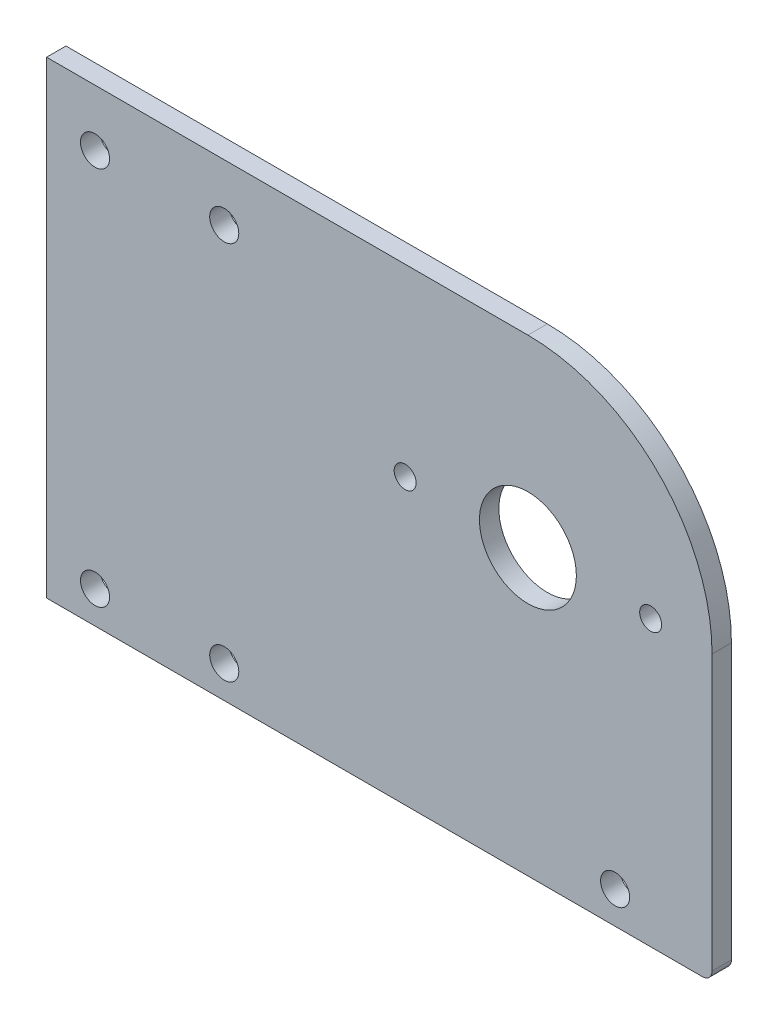
SolidWorks part; units mm, degrees
material "普通碳钢"
ref_plane "前视基准面" through (0, 0, 0) normal (0, 0, 1) x (1, 0, 0)
ref_plane "上视基准面" through (0, 0, 0) normal (0, 1, 0) x (1, 0, 0)
ref_plane "右视基准面" through (0, 0, 0) normal (1, 0, 0) x (0, 0, -1)
sketch "草图1" plane through (0, 0, 0) normal (0, 0, 1) x (1, 0, 0)
  line L0 (0, 72.5) -> (0, 0) construction
  line L1 (-103, 72.5) -> (103, 72.5)
  line L2 (-103, 72.5) -> (-103, -72.5)
  line L3 (-103, -72.5) -> (103, -72.5)
  line L4 (103, 72.5) -> (103, -72.5)
  line L5 (0, 0) -> (103, 0) construction
  dimension "D1" = 206
  dimension "D2" = 145
extrude "凸台-拉伸1" add sketch "草图1" along normal blind 6
sketch "草图2" plane through (0, 0, 6) normal (0, 0, 1) x (1, 0, 0)
  line L0 (103, 72.5) -> (-103, 72.5) construction
  line L1 (-103, -72.5) -> (-3, -72.5)
  line L2 (-103, -72.5) -> (-103, -7.5)
  line L3 (-103, -7.5) -> (-3, -7.5)
  line L4 (-3, -72.5) -> (-3, -7.5)
  dimension "D1" = 80
  dimension "D2" = 100
extrude "切除-拉伸1" [suppressed] cut sketch "草图2" against normal through all
sketch "草图3" plane through (0, 0, 6) normal (0, 0, 1) x (1, 0, 0)
  line L0 (103, 72.5) -> (-103, 72.5) construction
  line L1 (-103, 72.5) -> (-103, -72.5) construction
  circle A0 centre (-88, 55) radius 4.5
  circle A1 centre (-48, 55) radius 4.5
  circle A2 centre (-88, -62.5) radius 4.5
  circle A3 centre (-48, -62.5) radius 4.5
  dimension "D1" = 9
  dimension "D2" = 40
  dimension "D3" = 117.5
  dimension "D4" = 17.5
  dimension "D5" = 15
extrude "切除-拉伸2" cut sketch "草图3" against normal through all
sketch "草图4" plane through (0, 0, 6) normal (0, 0, 1) x (1, 0, 0)
  line L0 (103, 72.5) -> (-103, 72.5) construction
  line L2 (103, -72.5) -> (103, 72.5) construction
  circle A0 centre (46, 15.5) radius 15
  dimension "D1" = 30
  dimension "D3" = 57
  dimension "D2" = 57
extrude "切除-拉伸3" cut sketch "草图4" against normal through all
fillet "圆角1" radius 57 1 edges at (103, 72.5, 3)
fillet "圆角2" [suppressed] radius 10
fillet "圆角3" [suppressed] radius 10
sketch "草图5" plane through (0, 0, 6) normal (0, 0, 1) x (1, 0, 0)
  line L0 (46, 72.5) -> (-103, 72.5) construction
  line L1 (103, -72.5) -> (103, 15.5) construction
  circle A0 centre (88, 61) radius 2.75
  dimension "D1" = 11.5
  dimension "D2" = 5.5
  dimension "D3" = 15
extrude "切除-拉伸4" [suppressed] cut sketch "草图5" against normal through all
hole_wizard "M8 螺纹孔1" positions "草图7" profile "草图6" tap size "M8" standard "Gb" end condition through all
sketch "草图7" plane through (0, 0, 6) normal (0, 0, 1) x (1, 0, 0)
  line L0 (46, 41.9926) -> (46, 15.5) construction
  line L1 (46, 15.5) -> (88.8291, 15.5) construction
  point P0 (8, 15.5)
  dimension "D1" = 38
cosmetic thread "孔螺蚊线1" parameters "D2"=8
sketch "草图6" plane through (8, 15.5, 6) normal (1, 0, 0) x (0, -1, 0)
  line L0 (0, 0) -> (0, 6)
  line L1 (0, 6) -> (3.4, 6)
  line L2 (3.4, 6) -> (3.4, 0)
  line L5 (3.4, 0) -> (0, 0)
  line L11 (0, -6.35) -> (0, 107.95) construction
  dimension "通孔螺纹孔钻头直径" = 6.8
  dimension "通孔螺纹孔钻头深度" = 6
pattern_circular "阵列(圆周)1" count 2 over 360 about axis through (46, 15.5, 0) along (0, 0, 1) of "M8 螺纹孔1"
sketch "草图8" plane through (0, 0, 6) normal (0, 0, 1) x (1, 0, 0)
  line L1 (103, -72.5) -> (98, -72.5)
  line L2 (103, -72.5) -> (103, -27.5)
  line L3 (103, -27.5) -> (98, -27.5)
  line L4 (98, -72.5) -> (98, -27.5)
  dimension "D1" = 5
  dimension "D2" = 45
extrude "切除-拉伸5" [suppressed] cut sketch "草图8" against normal through all
hole_wizard "M4 螺纹孔1" positions "草图10" profile "草图9" tap size "M4" standard "Iso"
sketch "草图10" [suppressed] plane through (98, 0, 0) normal (1, 0, 0) x (0, 0, -1)
  line L0 (-4, -72.5) -> (-4, -23.5819) construction
  line L1 (0, -72.5) -> (-8, -72.5) construction
  point P0 (-4, -62.5)
  point P2 (-4, -37.5)
  dimension "D1" = 25
  dimension "D2" = 10
sketch "草图9" plane through (98, -62.5, 4) normal (0, 1, 0) x (0, 0, -1)
  line L0 (0, 0) -> (0, 12.4914)
  line L1 (0, 12.4914) -> (1.65, 11.5)
  line L2 (1.65, 11.5) -> (1.65, 0)
  line L5 (1.65, 0) -> (0, 0)
  line L10 (0, 12.4914) -> (-1.65, 11.5) construction
  line L11 (0, -6.35) -> (0, 107.95) construction
  dimension "螺纹孔钻头直径" = 3.3
  dimension "螺纹孔钻头深度" = 11.5
  dimension "导头角度" = 118
cosmetic thread "孔螺蚊线2" [suppressed] parameters "D1"=8, "D2"=4
cosmetic thread "孔螺蚊线3" [suppressed] parameters "D1"=8, "D2"=4
fillet "圆角4" [suppressed] radius 3
sketch "草图11" plane through (0, 0, 6) normal (0, 0, 1) x (1, 0, 0)
  line L0 (-103, -72.5) -> (103, -72.5) construction
  line L1 (103, -72.5) -> (103, 15.5) construction
  circle A0 centre (73, -62.5) radius 4.5
  dimension "D1" = 10
  dimension "D2" = 9
  dimension "D3" = 30
extrude "切除-拉伸6" cut sketch "草图11" against normal through all
fillet "圆角5" radius 3 1 edges at (103, -72.5, 3)
